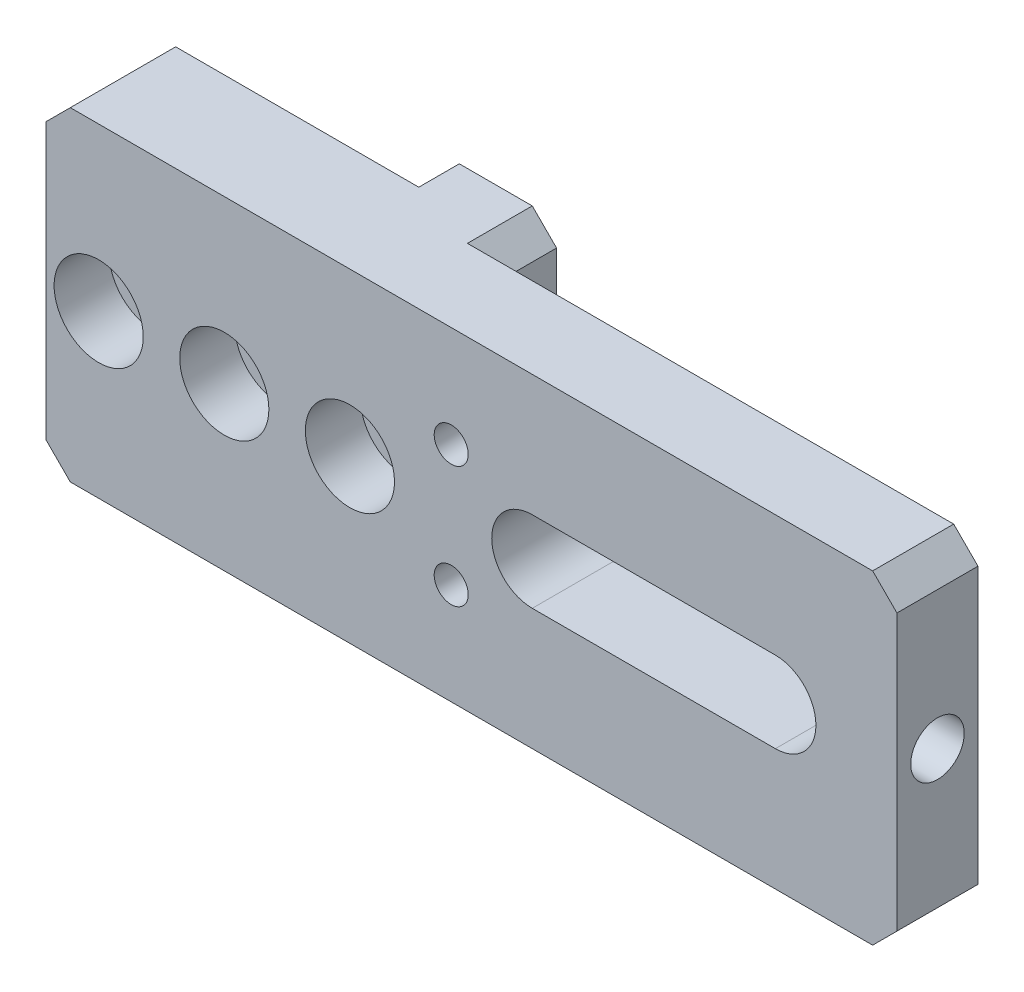
SolidWorks part; units mm, degrees
ref_plane "前视基准面" through (0, 0, 0) normal (0, 0, 1) x (1, 0, 0)
ref_plane "上视基准面" through (0, 0, 0) normal (0, 1, 0) x (1, 0, 0)
ref_plane "右视基准面" through (0, 0, 0) normal (1, 0, 0) x (0, 0, -1)
sketch "草图1" plane through (0, 0, 0) normal (0, 0, 1) x (1, 0, 0)
  line L1 (-52.5, -20) -> (52.5, -20)
  line L2 (-52.5, -20) -> (-52.5, 20)
  line L3 (-52.5, 20) -> (52.5, 20)
  line L4 (52.5, -20) -> (52.5, 20)
  line L5 (-52.5, -20) -> (52.5, 20) construction
  line L6 (-52.5, 20) -> (52.5, -20) construction
  point P0 (0, 0)
  dimension "D1" = 40
  dimension "D2" = 105
extrude "凸台-拉伸1" add sketch "草图1" along normal blind 18
sketch "草图2" plane through (0, 0, 0) normal (0, 0, -1) x (-1, 0, 0)
  line L0 (52.5, -20) -> (-52.5, -20) construction
  line L1 (52.5, 20) -> (22.5, 20)
  line L2 (52.5, 20) -> (52.5, -20)
  line L3 (52.5, -20) -> (22.5, -20)
  line L4 (22.5, 20) -> (22.5, -20)
  dimension "D1" = 30
extrude "切除-拉伸1" cut sketch "草图2" against normal blind 5
sketch "草图3" plane through (0, 0, 0) normal (0, 0, -1) x (-1, 0, 0)
  line L0 (22.5, -20) -> (-52.5, -20) construction
  line L1 (-52.5, 20) -> (7.5, 20)
  line L2 (-52.5, 20) -> (-52.5, -20)
  line L3 (-52.5, -20) -> (7.5, -20)
  line L4 (7.5, 20) -> (7.5, -20)
  dimension "D1" = 60
extrude "切除-拉伸2" cut sketch "草图3" against normal blind 8
hole_wizard "打孔尺寸(%根据)内六角圆柱头螺钉的类型1" positions "草图4" profile "草图5" counterbore size "M6" standard "GB" end condition through all
sketch "草图4" plane through (0, 0, 18) normal (0, 0, 1) x (1, 0, 0)
  line L0 (0, 0) -> (-15, 0) construction
  line L1 (-52.5, 20) -> (-52.5, -20) construction
  point P0 (-46, 0)
  point P2 (-30.5, 0)
  point P4 (-15, 0)
  dimension "D1" = 37.5
  dimension "D2" = 15.5
  dimension "D3" = 15.5
sketch "草图5" plane through (-46, 0, 18) normal (1, 0, 0) x (0, -1, 0)
  line L0 (0, 0) -> (0, 18)
  line L1 (0, 18) -> (3.3, 18)
  line L3 (3.3, 18) -> (3.3, 6.8)
  line L4 (3.3, 6.8) -> (5.5, 6.8)
  line L5 (5.5, 6.8) -> (5.5, 0)
  line L7 (5.5, 0) -> (0, 0)
  line L11 (0, -6.35) -> (0, 107.95) construction
  dimension "通孔孔直径" = 6.6
  dimension "通孔孔深度" = 18
  dimension "柱形沉头孔直径" = 11
  dimension "柱形沉头孔深度" = 6.8
sketch "草图6" plane through (0, 0, 0) normal (0, 0, -1) x (-1, 0, 0)
  circle A0 centre (15, 0) radius 5
  dimension "D1" = 10
extrude "切除-拉伸3" cut sketch "草图6" against normal blind 2
chamfer "倒角1" distance 3 angle 45 8 edges at (-22.5, -20, 2.5) (-7.5, -20, 4) (-7.5, 20, 4) (-22.5, 20, 2.5) (-52.5, 20, 11.5) (-52.5, -20, 11.5) (52.5, -20, 13) (52.5, 20, 13)
sketch "草图7" plane through (0, 0, 18) normal (0, 0, 1) x (1, 0, 0)
  line L0 (7.5, 0) -> (37.5, 0) construction
  line L1 (7.5, 5) -> (37.5, 5)
  line L2 (7.5, -5) -> (37.5, -5)
  line L3 (52.5, 0) -> (22.5, 0) construction
  line L4 (52.5, -17) -> (52.5, 17) construction
  arc A0 (7.5, 5) -> (7.5, -5) centre (7.5, 0) ccw
  arc A1 (37.5, -5) -> (37.5, 5) centre (37.5, 0) ccw
  point P2 (22.5, 0)
  point P12 (0, 0)
  point P13 (0, 0)
  dimension "D3" = 15
  dimension "D1" = 10
  dimension "D2" = 30
extrude "切除-拉伸4" cut sketch "草图7" against normal through all
hole_wizard "M6 间隙孔1" positions "草图8" profile "草图10" hole size "M6" standard "GB"
sketch "草图8" plane through (52.5, 0, 0) normal (1, 0, 0) x (0, 0, -1)
  line L0 (-8, 0) -> (-18, 0) construction
  line L1 (-8, 17) -> (-8, -17) construction
  line L2 (-18, -17) -> (-18, 17) construction
  point P0 (-13, 0)
  point P10 (-12.25, 0)
sketch "草图10" plane through (52.5, 0, 13) normal (0, 1, 0) x (0, 0, -1)
  line L0 (0, 0) -> (0, 10)
  line L1 (0, 10) -> (3.3, 10)
  line L2 (3.3, 10) -> (3.3, 0)
  line L5 (3.3, 0) -> (0, 0)
  line L11 (0, -6.35) -> (0, 107.95) construction
  dimension "通孔孔直径" = 6.6
  dimension "通孔孔深度" = 10
hole_wizard "M5 螺纹孔1" positions "草图11" profile "草图12" tap size "M5" standard "GB" end condition through all
sketch "草图11" plane through (0, 0, 18) normal (0, 0, 1) x (1, 0, 0)
  line L0 (-52.5, 17) -> (-52.5, -17) construction
  line L1 (0, 0) -> (-52.5, 0) construction
  point P0 (-2.5, 7.5)
  point P2 (-2.5, -7.5)
  dimension "D1" = 50
  dimension "D2" = 15
sketch "草图12" plane through (-2.5, 7.5, 18) normal (1, 0, 0) x (0, -1, 0)
  line L0 (0, 0) -> (0, 18)
  line L1 (0, 18) -> (2.1, 18)
  line L2 (2.1, 18) -> (2.1, 0)
  line L5 (2.1, 0) -> (0, 0)
  line L11 (0, -6.35) -> (0, 107.95) construction
  dimension "通孔螺纹孔钻头直径" = 4.2
  dimension "通孔螺纹孔钻头深度" = 18
cosmetic thread "孔螺蚊线1" parameters "D2"=5
cosmetic thread "孔螺蚊线2" parameters "D2"=5
